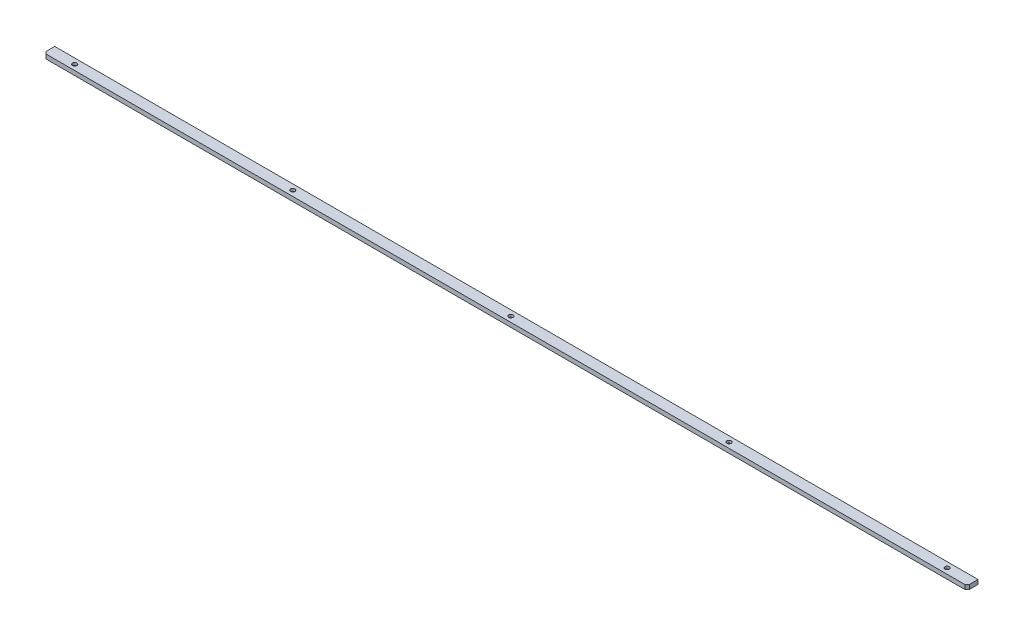
from build123d import *

# Parameters (mm, degrees)
SKETCH_1_W                = 1270
SKETCH_1_H                = 15
EXTRUDE_1_DEPTH           = 3
CHAMFER_1_SIZE            = 3
HOLE_WIZARD_1_D           = 3.4
HOLE_WIZARD_1_CBORE_D     = 6
HOLE_WIZARD_1_CBORE_DEPTH = 3.4


with BuildPart() as part:
    # 草图1 → 凸台-拉伸1 (new, symmetric)
    with BuildSketch(Plane(origin=(0, 0, 0), x_dir=(1, 0, 0), z_dir=(0, 1, 0))):
        Rectangle(SKETCH_1_W, SKETCH_1_H)
    extrude(amount=EXTRUDE_1_DEPTH, both=True)

    # 倒角1
    chamfer_1_edges = [part.edges().sort_by_distance(p)[0] for p in [
        (635, 0, 7.5),
        (-635, 0, 7.5),
    ]]
    chamfer(chamfer_1_edges, length=CHAMFER_1_SIZE)

    # 打孔尺寸(%根据)内六角圆柱头螺钉的类型1 (through all)
    with Locations(Plane(origin=(0, 3, 0), x_dir=(1, 0, 0), z_dir=(0, 1, 0))):
        with Locations((-600, 0), (-300, 0), (0, 0), (300, 0), (600, 0)):
            CounterBoreHole(HOLE_WIZARD_1_D / 2, HOLE_WIZARD_1_CBORE_D / 2, HOLE_WIZARD_1_CBORE_DEPTH)


solid = part.part
